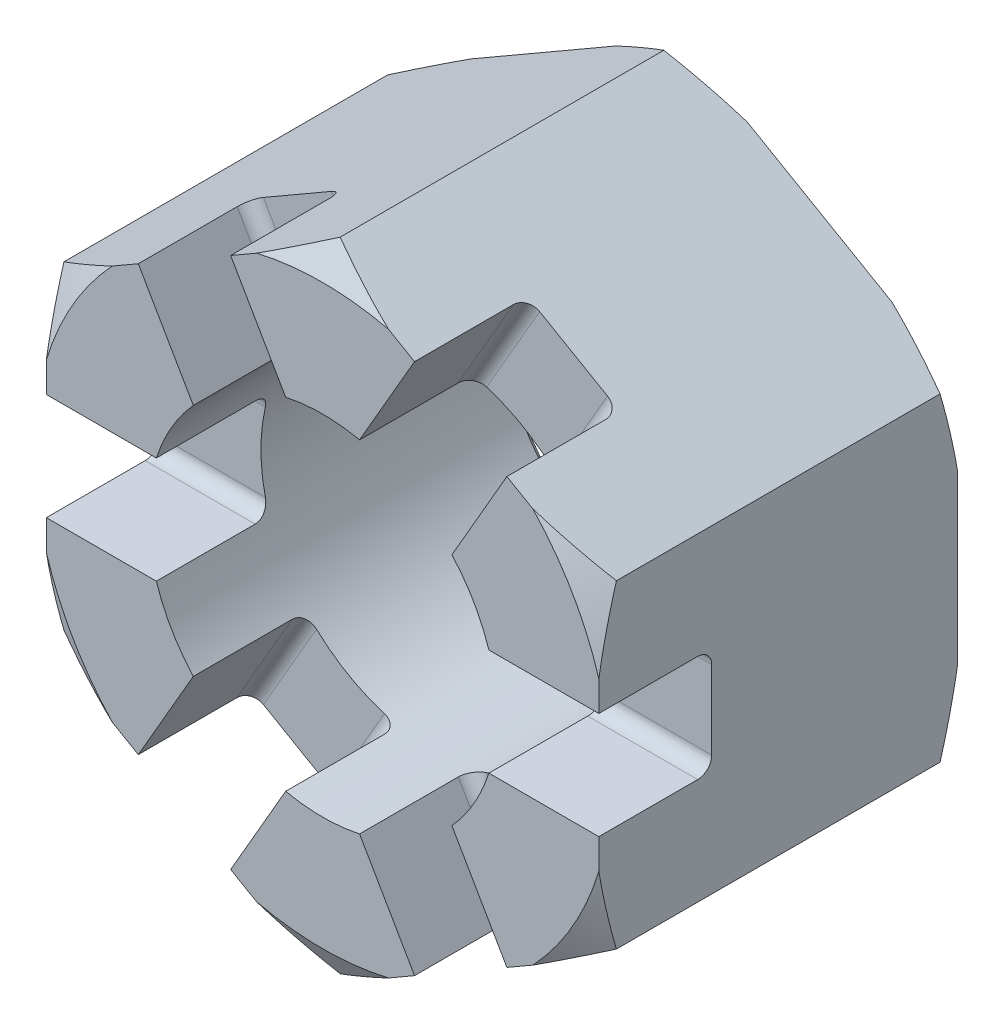
from build123d import *

# Parameters (mm, degrees)
SKETCH1_R          = 13.9175
BASE_EXTRUDE_DEPTH = 28.6
SKETCH2_OUTSIDE_W  = 217.06
SKETCH2_OUTSIDE_H  = 223.872
SKETCH2_OUTSIDE_R  = 23
CUT_EXTRUDE1_DEPTH = 45.149899136
CUT_EXTRUDE1_DRAFT = -60
SKETCH3_OUTSIDE_W  = 217.06
SKETCH3_OUTSIDE_H  = 223.872
SKETCH3_OUTSIDE_R  = 23
CUT_EXTRUDE2_DEPTH = 45.149899136
CUT_EXTRUDE2_DRAFT = -60
CUT_EXTRUDE3_DEPTH = 59.34108758
CIRPATTERN1_COUNT  = 3
CHAMFER1_SIZE      = 0.478571429


with BuildPart() as part:
    # Sketch1 → Base-Extrude (new body)
    with BuildSketch(Plane.XY):
        Polygon((0, 25.425), (-22.018695891, 12.7125), (-22.018695891, -12.7125), (0, -25.425), (22.018695891, -12.7125), (22.018695891, 12.7125), align=None)
        Circle(SKETCH1_R, mode=Mode.SUBTRACT)
    extrude(amount=BASE_EXTRUDE_DEPTH)


with BuildPart() as cut_extrude1_tool:
    # Sketch2 outside → Cut-Extrude1 (with draft: the straight prism first)
    with BuildSketch(Plane(origin=(0, 0, 0), x_dir=(-1, 0, 0), z_dir=(0, 0, -1))):
        Rectangle(SKETCH2_OUTSIDE_W, SKETCH2_OUTSIDE_H)
        Circle(SKETCH2_OUTSIDE_R, mode=Mode.SUBTRACT)
    extrude(amount=-CUT_EXTRUDE1_DEPTH)
    # Cut-Extrude1: the draft: its side faces are tilted about the plane it starts from
    cut_extrude1_sides = [cut_extrude1_tool.faces().sort_by_distance(p)[0] for p in [
        (0, -111.936, 22.574949568),
        (-108.53, 0, 22.574949568),
        (0, 111.936, 22.574949568),
        (108.53, 0, 22.574949568),
        (23, 0, 22.574949568),
    ]]
    draft(cut_extrude1_sides, Plane(origin=(0, 0, 0), x_dir=(-1, 0, 0), z_dir=(0, 0, -1)), CUT_EXTRUDE1_DRAFT)


with BuildPart() as part_1:
    add(part.part)

    # Cut-Extrude1: cut by cut_extrude1_tool
    add(cut_extrude1_tool.part, mode=Mode.SUBTRACT)


with BuildPart() as cut_extrude2_tool:
    # Sketch3 outside → Cut-Extrude2 (with draft: the straight prism first)
    with BuildSketch(Plane.XY.offset(28.6)):
        Rectangle(SKETCH3_OUTSIDE_W, SKETCH3_OUTSIDE_H)
        Circle(SKETCH3_OUTSIDE_R, mode=Mode.SUBTRACT)
    extrude(amount=-CUT_EXTRUDE2_DEPTH)
    # Cut-Extrude2: the draft: its side faces are tilted about the plane it starts from
    cut_extrude2_sides = [cut_extrude2_tool.faces().sort_by_distance(p)[0] for p in [
        (0, -111.936, 6.025050432),
        (108.53, 0, 6.025050432),
        (0, 111.936, 6.025050432),
        (-108.53, 0, 6.025050432),
        (-23, 0, 6.025050432),
    ]]
    draft(cut_extrude2_sides, Plane.XY.offset(28.6), CUT_EXTRUDE2_DRAFT)


with BuildPart() as part_2:
    add(part_1.part)

    # Cut-Extrude2: cut by cut_extrude2_tool
    add(cut_extrude2_tool.part, mode=Mode.SUBTRACT)

    # Sketch6 → Cut-Extrude3 (cut, through all)
    with BuildSketch(Plane(origin=(22.018695891, 0, 0), x_dir=(0, 0, -1), z_dir=(1, 0, 0))):
        with BuildLine():
            Line((-28.6, -4.25), (-28.6, 4.25))
            Line((-28.6, 4.25), (-20.725, 4.25))
            ThreePointArc((-20.725, 4.25), (-19.929504871, 3.920495129), (-19.6, 3.125))
            Line((-19.6, 3.125), (-19.6, -3.125))
            ThreePointArc((-19.6, -3.125), (-19.929504871, -3.920495129), (-20.725, -4.25))
            Line((-20.725, -4.25), (-28.6, -4.25))
        make_face()
    cut_extrude3 = extrude(amount=-CUT_EXTRUDE3_DEPTH, mode=Mode.SUBTRACT)

    # CirPattern1: Cut-Extrude3 ×3 about axis
    cirpattern1_axis = Axis((0, 0, 0), (0, 0, 1))
    for i in range(1, CIRPATTERN1_COUNT):
        add(cut_extrude3.rotate(cirpattern1_axis, i * 360 / CIRPATTERN1_COUNT), mode=Mode.SUBTRACT)

    # Chamfer1
    chamfer1_edges = [part_2.edges().sort_by_distance(p)[0] for p in [
        (-13.9175, 0, 0),
    ]]
    chamfer(chamfer1_edges, length=CHAMFER1_SIZE)


solid = part_2.part
